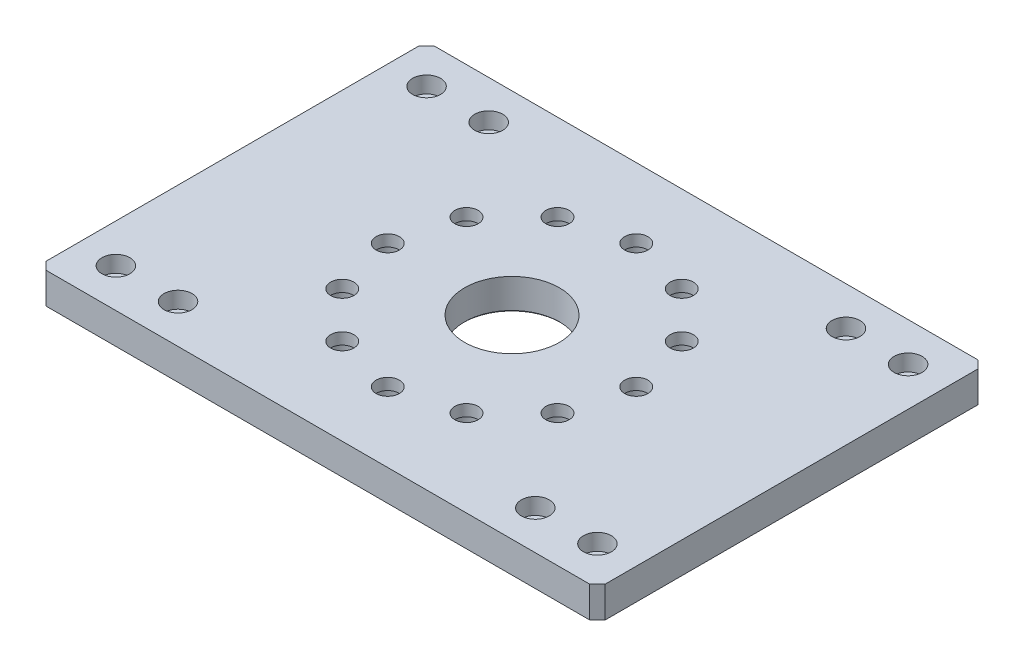
SolidWorks part; units mm, degrees
material "Q235A"
ref_plane "前视基准面" through (0, 0, 0) normal (0, 0, 1) x (1, 0, 0)
ref_plane "上视基准面" through (0, 0, 0) normal (0, 1, 0) x (1, 0, 0)
ref_plane "右视基准面" through (0, 0, 0) normal (1, 0, 0) x (0, 0, -1)
ref_plane "基准面1" through (0, 63, 0) normal (0, -1, 0) x (1, 0, 0)
sketch "草图1" plane through (0, 63, 0) normal (0, -1, 0) x (1, 0, 0)
  line L0 (135.1, -120) -> (135.1, -370)
  line L1 (135.1, -370) -> (495.1, -370)
  line L2 (495.1, -370) -> (495.1, -120)
  line L3 (495.1, -120) -> (135.1, -120)
extrude "凸台-拉伸1" add sketch "草图1" against normal blind 20
hole_wizard "M10 六角凹头螺钉的柱形沉头孔1" positions "草图3" profile "草图2" counterbore size "M10" standard "ISO" end condition through all
sketch "草图3" plane through (0, 83, 0) normal (0, -1, 0) x (-1, 0, 0)
  point P0 (-470.1, 345)
  point P1 (-430.1, 345)
  point P2 (-470.1, 145)
  point P3 (-430.1, 145)
  point P4 (-200.1, 145)
  point P5 (-200.1, 345)
  point P6 (-160.1, 145)
  point P7 (-160.1, 345)
sketch "草图2" plane through (470.1, 83, -345) normal (1, 0, 0) x (0, 0, 1)
  line L0 (0, 0) -> (0, 20)
  line L1 (0, 20) -> (6, 20)
  line L3 (6, 20) -> (6, 10.6)
  line L4 (6, 10.6) -> (9, 10.6)
  line L5 (9, 10.6) -> (9, 0)
  line L7 (9, 0) -> (0, 0)
  line L11 (0, -6.35) -> (0, 107.95) construction
  dimension "通孔孔直径" = 12
  dimension "通孔孔深度" = 20
  dimension "柱形沉头孔直径" = 18
  dimension "柱形沉头孔深度" = 10.6
hole_wizard "M52 间隙孔1" positions "草图5" profile "草图4" hole size "M52" standard "ANSI Metric"
sketch "草图5" plane through (0, 63, 0) normal (0, -1, 0) x (-1, 0, 0)
  point P0 (-315.1, 245)
sketch "草图4" plane through (315.1, 63, -245) normal (1, 0, 0) x (0, 0, -1)
  line L0 (0, 0) -> (0, 20)
  line L1 (0, 20) -> (30.5, 20)
  line L2 (30.5, 20) -> (30.5, 0)
  line L5 (30.5, 0) -> (0, 0)
  line L11 (0, -6.35) -> (0, 107.95) construction
  dimension "通孔孔直径" = 61
  dimension "通孔孔深度" = 20
hole_wizard "M12 六角凹头螺钉的柱形沉头孔1" positions "草图7" profile "草图6" counterbore size "M12" standard "ISO" end condition through all
sketch "草图7" plane through (0, 63, 0) normal (0, -1, 0) x (-1, 0, 0)
  point P0 (-245.818, 205)
  point P1 (-275.1, 175.718)
  point P2 (-315.1, 165)
  point P3 (-355.1, 175.718)
  point P4 (-384.382, 205)
  point P5 (-395.1, 245)
  point P6 (-384.382, 285)
  point P7 (-355.1, 314.282)
  point P8 (-315.1, 325)
  point P9 (-275.1, 314.282)
  point P10 (-245.818, 285)
  point P11 (-235.1, 245)
sketch "草图6" plane through (245.818, 63, -205) normal (1, 0, 0) x (0, 0, -1)
  line L0 (0, 0) -> (0, 20)
  line L1 (0, 20) -> (7.5, 20)
  line L3 (7.5, 20) -> (7.5, 12.6)
  line L4 (7.5, 12.6) -> (10, 12.6)
  line L5 (10, 12.6) -> (10, 0)
  line L7 (10, 0) -> (0, 0)
  line L11 (0, -6.35) -> (0, 107.95) construction
  dimension "通孔孔直径" = 15
  dimension "通孔孔深度" = 20
  dimension "柱形沉头孔直径" = 20
  dimension "柱形沉头孔深度" = 12.6
chamfer "倒角1" distance 1 angle 45 1 edges at (315.1, 63, -275.5)
chamfer "倒角2" distance 5 angle 45 4 edges at (495.1, 73, -120) (495.1, 73, -370) (135.1, 73, -370) (135.1, 73, -120)
